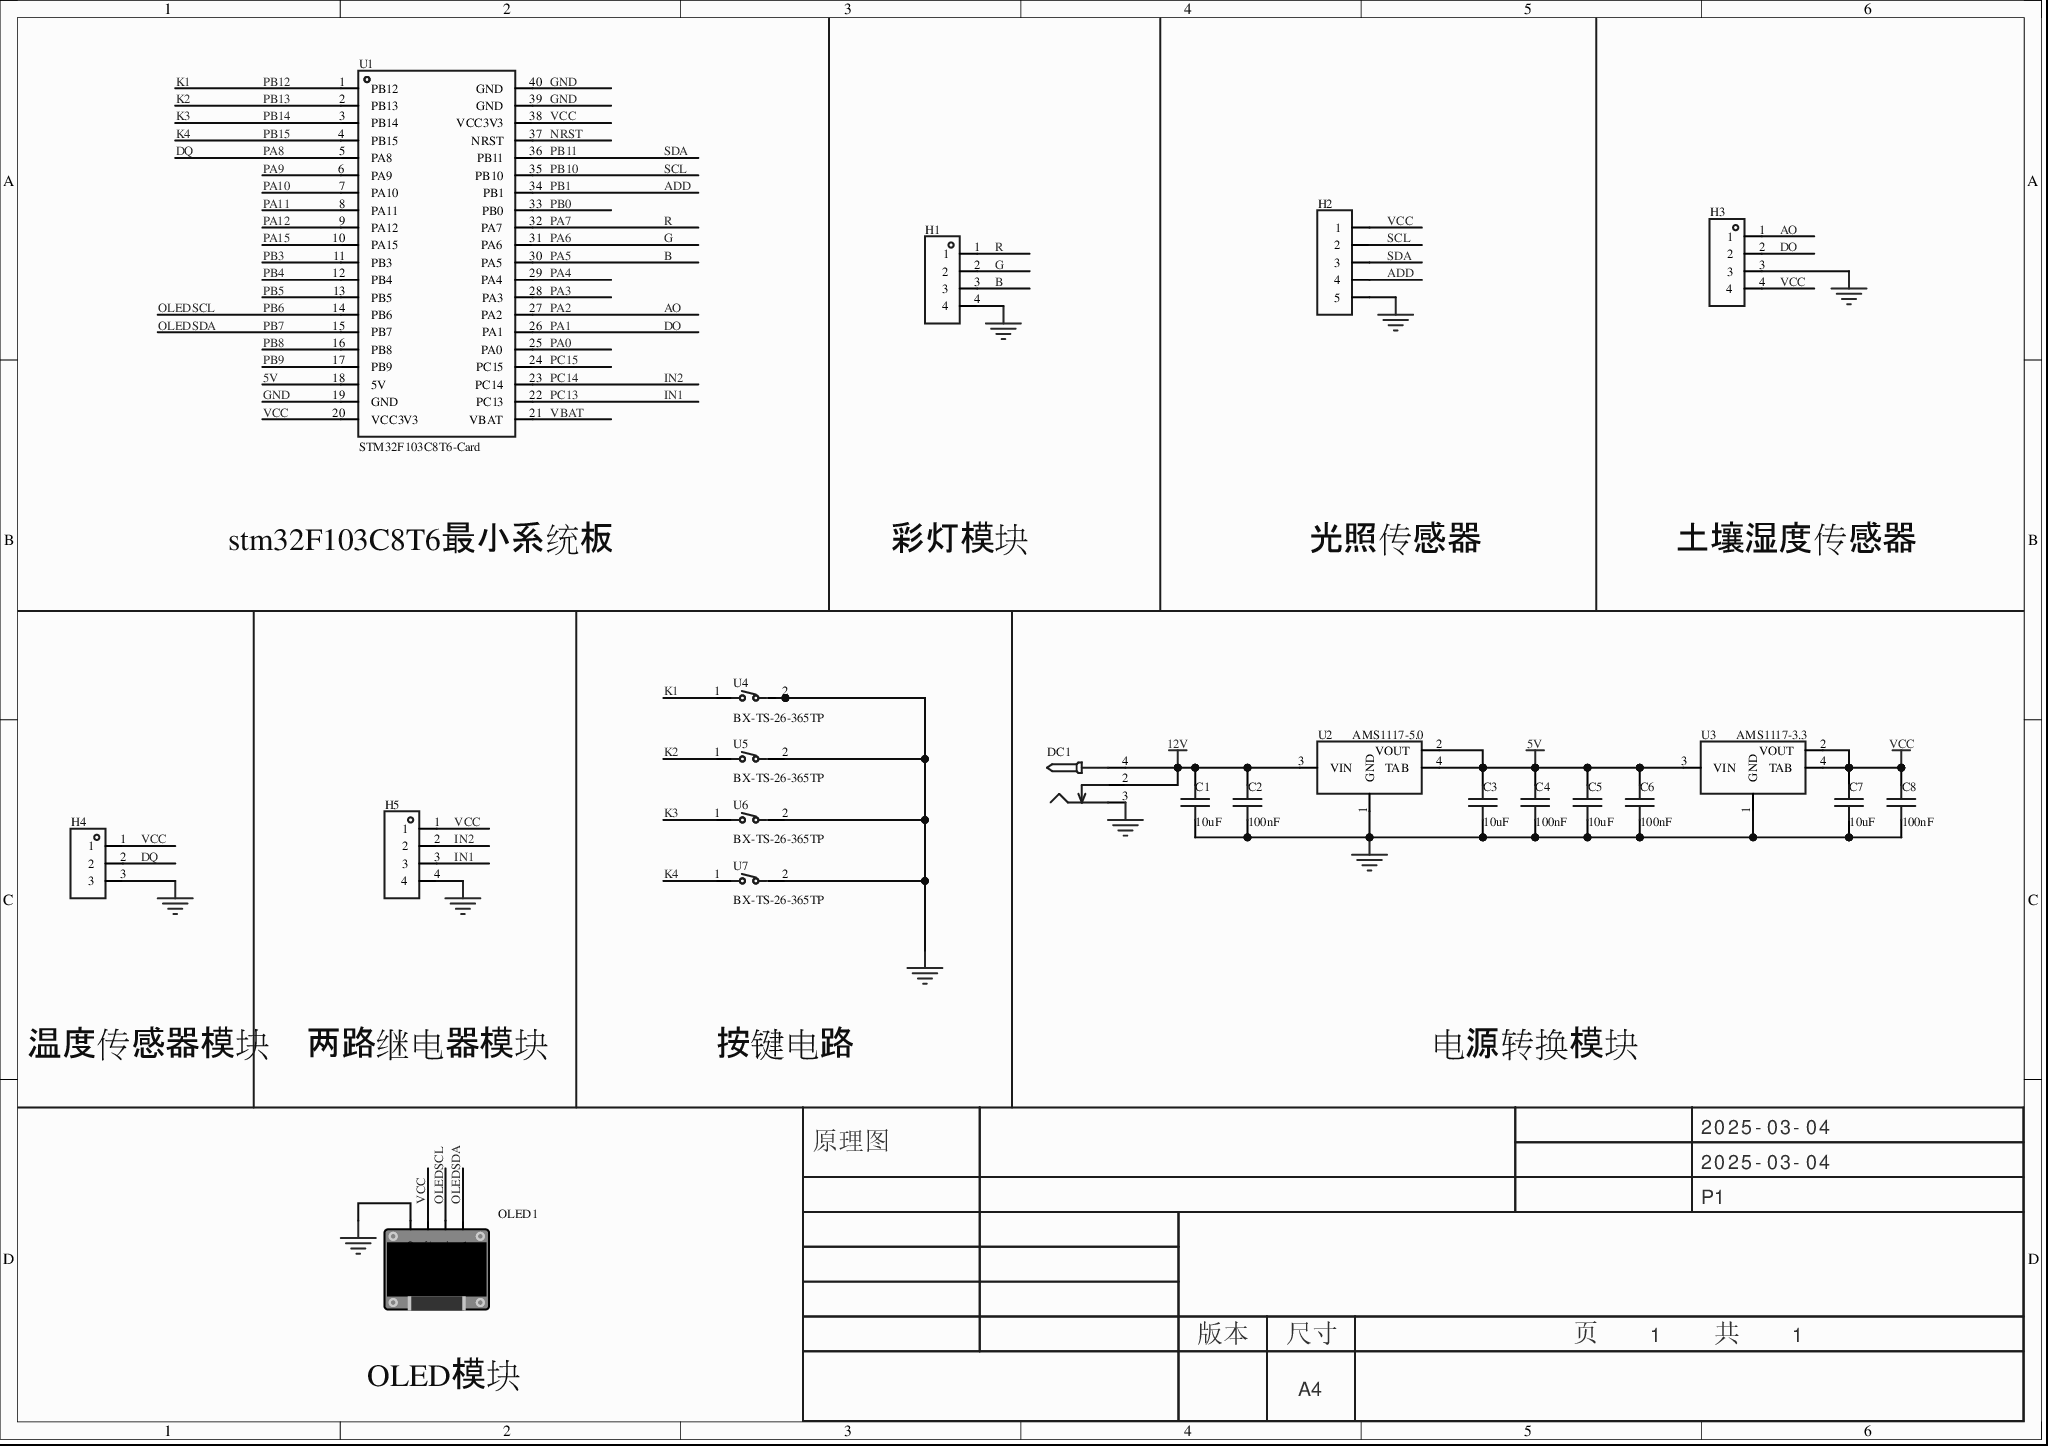
[diagram p0: MISC51501-3.schdoc]
# Altium project MISC51501-2.PrjPcb
1 sheet, 22 parts. Net scope: global (net labels, ports and power ports of the same name join across sheets).
Board file: MISC51501.pcbdoc

## Sheet MISC51501-3.schdoc
size 297 x 209 mm; Version: V1.0; @Project Name: MISC51501; @Page Count: 1; @Update Date: 2025-03-04; @Create Date: 2025-03-04; @Schematic Name: MISC51501; @Page No: 1; @Create Time: 18:09:00; @Update Time: 18:09:00; @Board Name: MISC51501

### Parts
C1  10uF  [C0805]
C2  100nF  [C0805]
C3  10uF  [C0805]
C4  100nF  [C0805]
C5  10uF  [C0805]
C6  100nF  [C0805]
C7  10uF  [C0805]
C8  100nF  [C0805]
DC1  (no value)  [DC-2.0]
H1  (no value)  [HDR-TH_4P-P2.54-V-F]
H2  (no value)  [HDR-TH_5P-P2.54-V-F]
H3  (no value)  [HDR-TH_4P-P2.54-V-F]
H4  (no value)  [HDR-TH_3P-P2.54-V-F]
H5  (no value)  [HDR-TH_4P-P2.54-V-F]
OLED1  (no value)  [0.96OLED_4P]
U1  STM32F103C8T6-Card  [CONN-TH_L53.3-W22.9_STM32F103C8T6-CARD]
U2  AMS1117-5.0  [SOT_223]
U3  AMS1117-3.3  [SOT_223]
U4  BX-TS-26-365TP  [KEY-SMD_L6.0-W3.5-LS8.0-1]
U5  BX-TS-26-365TP  [KEY-SMD_L6.0-W3.5-LS8.0-1]
U6  BX-TS-26-365TP  [KEY-SMD_L6.0-W3.5-LS8.0-1]
U7  BX-TS-26-365TP  [KEY-SMD_L6.0-W3.5-LS8.0-1]

### Nets
5V: C3.2 C4.2 C5.2 C6.2 U1.18(5V) U2.2(VOUT) U2.4(TAB) U3.3(VIN)
12V: C1.2 C2.2 DC1.2 DC1.4 U2.3(VIN)
GND: C1.1 C2.1 C3.1 C4.1 C5.1 C6.1 C7.1 C8.1 DC1.3 H1.4 H2.5 H3.3 H4.3 H5.4 OLED1.1(GND) U1.19(GND) U1.39(GND) U1.40(GND) U2.1(GND) U3.1(GND) U4.2 U5.2 U6.2 U7.2
VCC: C7.2 C8.2 H2.1 H3.4 H4.1 H5.1 OLED1.2(VCC) U1.20(VCC3V3) U1.38(VCC3V3) U3.2(VOUT) U3.4(TAB)
ADD: H2.4 U1.34(PB1)  [also labelled PB1]
AO: H3.1 U1.27(PA2)  [also labelled PA2]
B: H1.3 U1.30(PA5)  [also labelled PA5]
DO: H3.2 U1.26(PA1)  [also labelled PA1]
DQ: H4.2 U1.5(PA8)  [also labelled PA8]
G: H1.2 U1.31(PA6)  [also labelled PA6]
IN1: H5.3 U1.22(PC13)  [also labelled PC13]
IN2: H5.2 U1.23(PC14)  [also labelled PC14]
K1: U1.1(PB12) U4.1  [also labelled PB12]
K2: U1.2(PB13) U5.1  [also labelled PB13]
K3: U1.3(PB14) U6.1  [also labelled PB14]
K4: U1.4(PB15) U7.1  [also labelled PB15]
NRST: U1.37(NRST)
OLEDSCL: OLED1.3(SCL) U1.14(PB6)  [also labelled PB6]
OLEDSDA: OLED1.4(SDA) U1.15(PB7)  [also labelled PB7]
PA0: U1.25(PA0)
PA3: U1.28(PA3)
PA4: U1.29(PA4)
PA7: H1.1 U1.32(PA7)  [also labelled R]
PA9: U1.6(PA9)
PA10: U1.7(PA10)
PA11: U1.8(PA11)
PA12: U1.9(PA12)
PA15: U1.10(PA15)
PB0: U1.33(PB0)
PB3: U1.11(PB3)
PB4: U1.12(PB4)
PB5: U1.13(PB5)
PB8: U1.16(PB8)
PB9: U1.17(PB9)
PB10: H2.2 U1.35(PB10)  [also labelled SCL]
PB11: H2.3 U1.36(PB11)  [also labelled SDA]
PC15: U1.24(PC15)
VBAT: U1.21(VBAT)

### Notes on the sheet
- stm32F103C8T6最小系统板
- 彩灯模块
- 光照传感器
- 土壤湿度传感器
- 温度传感器模块
- 两路继电器模块
- 按键电路
- 电源转换模块
- OLED模块
- 2025-03-04
- 原理图
- P1
- 版本
- 尺寸
- A4
- 页    1    共    1

### Library data of the parts
C1-C8 = CAP_0805: ConvertToPcb: yes; SymbolName: CapAcitance; ModelId: 1ba041120af144c991958decab20d241; ModelName: C0805_L2.0-W1.3-H1.3; ModelTransform: 78.74,51.181,0,0,0,0,0,0.0005,0; Device: CAP_0805; AddInBom: yes; Supplier Footprint: 0805; FootprintName: C0805
  C1 C3 C5 C7: Value: 10uF
  C2 C4 C6 C8: Value: 100nF
DC1 = DC-005_2.0: ConvertToPcb: yes; SymbolName: DC电源接口; ModelId: f5f20b8a2308479b936ba3c2698865bb0819f05c4eef4c71ace90d822a990e87; ModelName: DC-IN-TH_DC-5520-1; ModelTransform: 372.05,551.18,582.68,90,0,0,137.8,0,-149.61; Device: DC-005_2.0; AddInBom: yes; Supplier Footprint: 插件; FootprintName: DC-2.0
H1 H3 H5 = HDR-F_2.54_1x4P: Symbol: 2.54-1*4P母; ConvertToPcb: yes; ModelId: d187812051054f85879fcaa51a310d8e; ModelTransform: 419.6842,98.464,0,0,0,0,0,0,-118.11; Device: HDR-F_2.54_1x4P; AddInBom: yes; SupplierPart: C2718488; Supplier Footprint: 插件; FootprintName: HDR-TH_4P-P2.54-V-F; ModelName: HDR-TH_4P-P2.54-V-F
H2 = HDR-F_2.54_1x5P: Symbol: Header-Female-2.54_1x5; ConvertToPcb: yes; ModelId: f49cb6116a3d45e5a64915bf3e00773f; ModelTransform: 519.684,98.464,0,0,0,0,0,0,-124.016; Device: HDR-F_2.54_1x5P; AddInBom: yes; SupplierPart: C50950; Supplier Footprint: 插件; FootprintName: HDR-TH_5P-P2.54-V-F; ModelName: HDR-TH_5P-P2.54-V-F
H4 = HDR-F_2.54_1x3P: Symbol: PM254V-11-03-H85; ConvertToPcb: yes; ModelId: f3b3cc5aae9641bf9e56fc160cef875b; ModelName: HDR2.54-F-LI-1X3P; ModelTransform: 299.9994,100,0,0,0,0,0,0,-118.11; Device: HDR-F_2.54_1x3P; AddInBom: yes; SupplierPart: C541850; Supplier Footprint: 插件; FootprintName: HDR-TH_3P-P2.54-V-F
OLED1 = 0.96OLED模块_4P: ConvertToPcb: yes; ModelId: 79c000fdb68d45a296c2e9bedf4f9055; ModelTransform: 1393.69792,1318.895,0,0,0,0,0,-560.079,-137.795; Device: 0.96OLED模块_4P; AddInBom: yes; SymbolName: 0.96OLED模块_4P; FootprintName: 0.96OLED_4P; Supplier Footprint: 插件; ModelName: 0.96OLED_4P
U1 = STM32F103C8T6-Card: AddInBom: yes; Symbol: STM32F103C8T6-CARD; Device: STM32F103C8T6-Card; LCSC Part Name: STM32F103C8T6-Card; SupplierPart: C9900077949; ManufacturerPart: STM32F103C8T6-Card; Supplier Footprint: 插件; Supplier: LCSC; ConvertToPcb: yes; FootprintName: CONN-TH_L53.3-W22.9_STM32F103C8T6-CARD
U2 U3 = AMS1117: Symbol: AMS1117_OLD; AddInBom: yes; ModelId: 925194bf9823436183a3e0b978a8d0760819f05c4eef4c71ace90d822a990e87; ModelName: SOT-223-4P_L6.5-W3.5-H1.6-LS7.0-P2.30; ModelTransform: 279.84,255.85,68.86,90,0,0,0,0,0; Device: AMS1117; ConvertToPcb: yes; FootprintName: SOT_223; Supplier Footprint: SOT_223
U4-U7 = BX-TS-26-365TP: 电路结构:单刀单掷;按钮形状:矩形按钮;作用力:260gf;安装方式:立贴;开关长度:3mm;开关宽度:6mm;开关高度:5mm;带支架:不带;触点电流:50mA;额定电压(AC):250V;额定电压(DC):12V;绝缘电阻:100MΩ;机械寿命:10万次;; Manufacturer: Bossie(博锡); AddInBom: yes; ModelId: 51ffbe84bd744a4ab29d6010491911d6; ModelTransform: 314.96,137.795,0,0,0,0,0,0,0; Circuit: 单刀单掷; Actuator Style: 矩形按钮; Operating Force: 260gf; Switch Length: 3mm; Switch Width: 6mm; Switch Height: 5mm; Strike Gundam: 不带; Contact Current: 50mA; Voltage Rating (AC): 250V; Voltage Rating (DC): 12V; Insulation Resistance: 100MΩ; Actuator/Cap Color: 白色; Pin Style: 鸥翼型; Mechanical Life: 10万次; Symbol: BX-TS-26-365TP; Device: BX-TS-26-365TP; LCSC Part Name: 3x6x5贴片开关无定位; SupplierPart: C18078120; ManufacturerPart: BX-TS-26-365TP; Supplier Footprint: SMD,3.5x6mm; JLCPCB Part Class: 扩展库; Datasheet: https://atta.szlcsc.com/upload/public/pdf/source/20231017/C9E3A2AEFECBEA609D28A37A0FA3E654.pdf; Supplier: LCSC; ConvertToPcb: yes; FootprintName: KEY-SMD_L6.0-W3.5-LS8.0-1; ModelName: KEY-SMD_L6.0-W3.5-LS8.0-1; Mounting Style: 立贴; Operating Temperature: -30℃~+80℃